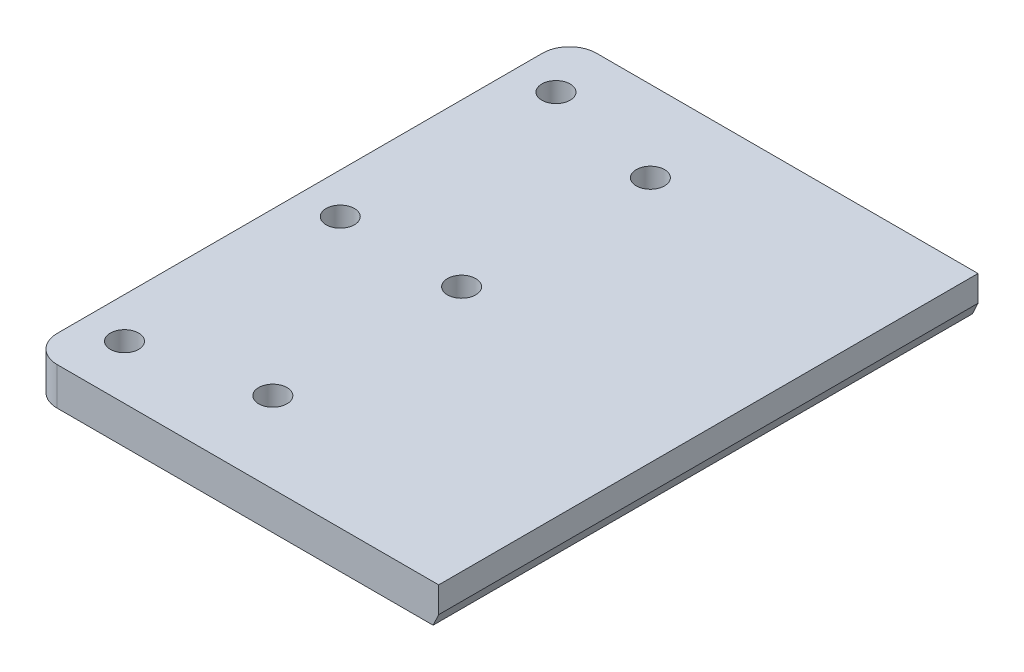
SolidWorks part; units mm, degrees
material "普通碳钢"
ref_plane "Front" through (0, 0, 0) normal (0, 0, 1) x (1, 0, 0)
ref_plane "Top" through (0, 0, 0) normal (0, 1, 0) x (1, 0, 0)
ref_plane "Right" through (0, 0, 0) normal (1, 0, 0) x (0, 0, -1)
sketch "Sketch1" plane through (0, 0, 0) normal (0, 1, 0) x (1, 0, 0)
  line L0 (0, 0) -> (102.7266, 0) construction
  line L1 (0, -100) -> (0, 100)
  line L2 (0, 100) -> (80, 100)
  line L4 (80, 100) -> (160, 100)
  line L5 (160, 100) -> (160, -100)
  line L6 (80, -100) -> (160, -100)
  line L8 (0, -100) -> (80, -100)
  point P14 (160, 0)
  dimension "D2" = 200
  dimension "D3" = 160
extrude "Boss-Extrude1" add sketch "Sketch1" along normal blind 14
fillet "Fillet1" radius 10 2 edges at (0, 7, -100) (0, 7, 100)
hole_wizard "Ø10.5 (10.5) Diameter Hole1" positions "Sketch2" profile "Sketch3" hole size "Ø10.5" standard "GB" end condition through all
sketch "Sketch2" plane through (0, 14, 0) normal (0, 1, 0) x (1, 0, 0)
  line L0 (0, 0) -> (60, 0) construction
  line L3 (60, 70) -> (60, 0) construction
  line L4 (60, 0) -> (60, -70) construction
  point P0 (60, 70)
  point P2 (60, -70)
  point P11 (60, 0)
  dimension "D2" = 140
  dimension "D3" = 60
sketch "Sketch3" plane through (60, 14, -70) normal (1, 0, 0) x (0, 0, 1)
  line L0 (0, 0) -> (0, 14)
  line L1 (0, 14) -> (5.25, 14)
  line L2 (5.25, 14) -> (5.25, 0)
  line L5 (5.25, 0) -> (0, 0)
  line L11 (0, -6.35) -> (0, 107.95) construction
  dimension "通孔孔直径" = 10.5
  dimension "通孔孔深度" = 14
hole_wizard "Ø10.5 (10.5) Diameter Hole2" positions "Sketch5" profile "Sketch6" hole size "Ø10.5" standard "GB" end condition through all
sketch "Sketch5" plane through (0, 14, 0) normal (0, 1, 0) x (1, 0, 0)
  line L0 (0, 0) -> (15, 0) construction
  line L2 (15, 55.868) -> (15, 80) construction
  line L3 (15, 80) -> (15, 0) construction
  line L4 (15, 0) -> (15, -80) construction
  circle A0 centre (60, 70) radius 5.25 construction
  point P0 (15, 80)
  point P2 (15, -80)
  point P16 (15, 0)
  dimension "D1" = 160
  dimension "D2" = 45
sketch "Sketch6" plane through (15, 14, -80) normal (1, 0, 0) x (0, 0, 1)
  line L0 (0, 0) -> (0, 14)
  line L1 (0, 14) -> (5.25, 14)
  line L2 (5.25, 14) -> (5.25, 0)
  line L5 (5.25, 0) -> (0, 0)
  line L11 (0, -6.35) -> (0, 107.95) construction
  dimension "通孔孔直径" = 10.5
  dimension "通孔孔深度" = 14
sketch "Sketch7" plane through (0, 0, 100) normal (0, 0, 1) x (1, 0, 0)
  line L0 (149.4345, 0) -> (160, 22.6577)
  line L1 (10, 0) -> (160, 0) construction
  line L2 (160, 14) -> (160, 0) construction
  line L3 (149.4345, 0) -> (160, 0)
  line L4 (160, 22.6577) -> (160, 0)
  dimension "D1" = 65
  dimension "D2" = 25
extrude "Cut-Extrude1" cut sketch "Sketch7" against normal through all
sketch "Sketch8" plane through (0, 0, 100) normal (0, 0, 1) x (1, 0, 0)
  line L0 (0, 0) -> (0, 14) construction
  line L1 (155.9629, 14) -> (151.5, 14)
  line L2 (155.9629, 14) -> (155.9629, -1.004)
  line L3 (155.9629, -1.004) -> (151.5, -1.004)
  line L4 (151.5, 14) -> (151.5, -1.004)
  dimension "D1" = 151.5
extrude "Cut-Extrude2" cut sketch "Sketch8" against normal through all
